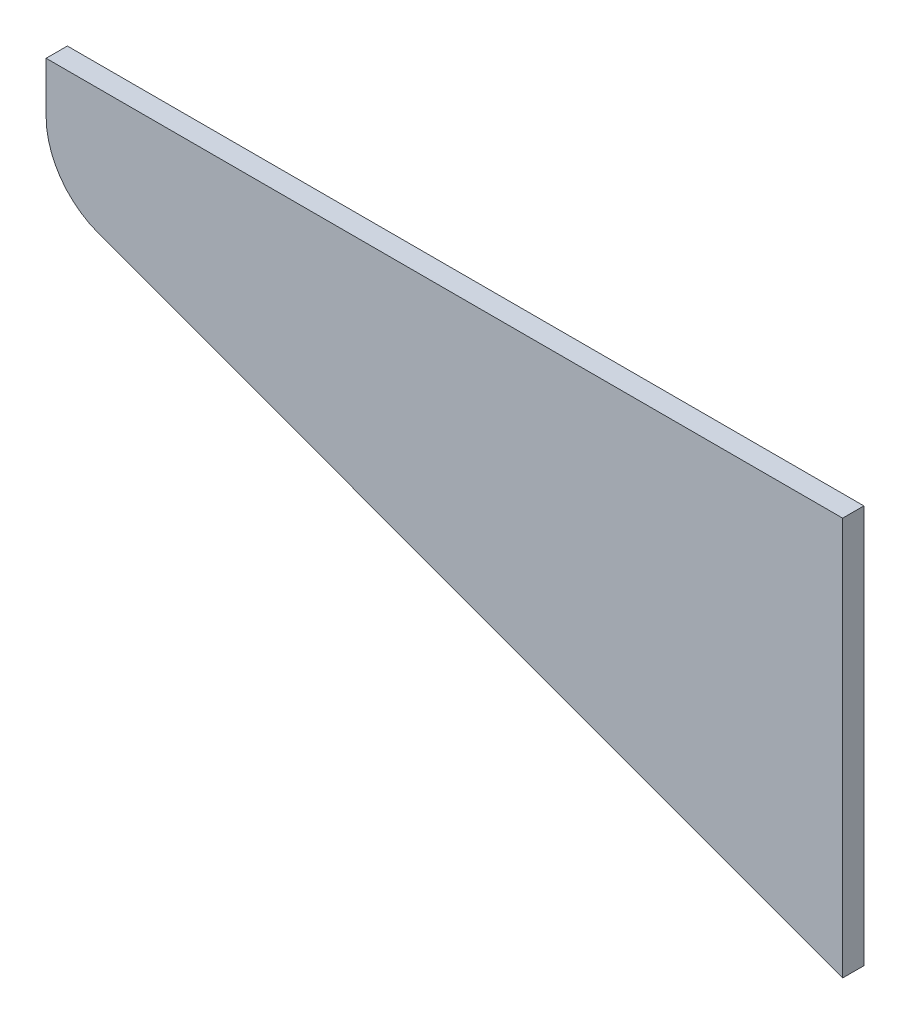
SolidWorks part; units mm, degrees
ref_plane "前视基准面" through (0, 0, 0) normal (0, 0, 1) x (1, 0, 0)
ref_plane "上视基准面" through (0, 0, 0) normal (0, 1, 0) x (1, 0, 0)
ref_plane "右视基准面" through (0, 0, 0) normal (1, 0, 0) x (0, 0, -1)
sketch "草图1" plane through (0, 0, 0) normal (0, 0, 1) x (1, 0, 0)
  line L0 (330, 0) -> (30, 0)
  line L1 (330, 0) -> (330, -150)
  line L2 (30, 0) -> (30, -19.0469)
  line L3 (49.6724, -47.2132) -> (330, -150)
  arc A0 (30, -19.0469) -> (49.6724, -47.2132) centre (60, -19.0469) ccw
  dimension "D1" = 30
extrude "凸台-拉伸2" add sketch "草图1" along normal blind 8
